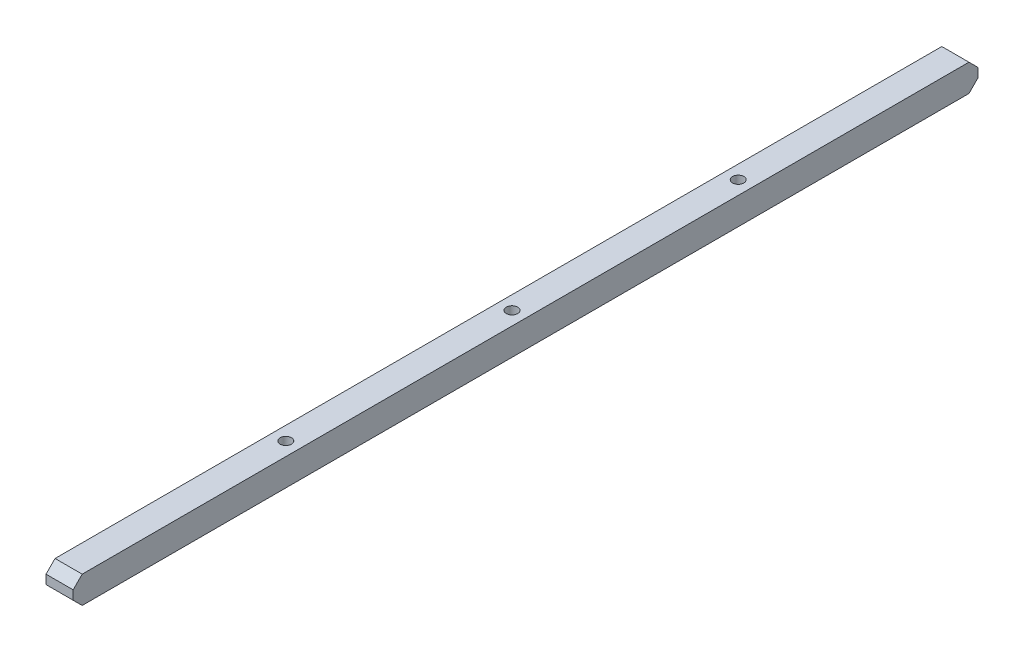
SolidWorks part; units mm, degrees
material "AISI 1045 钢，冷拔"
ref_plane "前视基准面" through (0, 0, 0) normal (0, 0, 1) x (1, 0, 0)
ref_plane "上视基准面" through (0, 0, 0) normal (0, 1, 0) x (1, 0, 0)
ref_plane "右视基准面" through (0, 0, 0) normal (1, 0, 0) x (0, 0, -1)
sketch "草图1" plane through (0, 0, 0) normal (0, 0, 1) x (1, 0, 0)
  line L1 (-3, 3) -> (3, 3)
  line L2 (-3, 3) -> (-3, -3)
  line L3 (-3, -3) -> (3, -3)
  line L4 (3, 3) -> (3, -3)
  line L5 (-3, 3) -> (3, -3) construction
  line L6 (-3, -3) -> (3, 3) construction
  point P0 (0, 0)
  dimension "D1" = 6
extrude "凸台-拉伸1" add sketch "草图1" along normal blind 200
sketch "草图2" plane through (0, 3, 0) normal (0, 1, 0) x (1, 0, 0)
  line L0 (0, 0) -> (0, -50) construction
  line L1 (0, -50) -> (0, -100) construction
  line L2 (0, -100) -> (0, -150) construction
  line L3 (0, -150) -> (0, -200) construction
  line L4 (3, -200) -> (-3, -200) construction
  dimension "D1" = 50
hole_wizard "M3 螺纹孔1" positions "3D草图1" profile "草图3" tap size "M3" standard "GB" end condition through all
sketch3d "3D草图1"
  point P0 (0, 3, 50)
  point P3 (0, 3, 100)
  point P6 (0, 3, 150)
sketch "草图3" plane through (0, 3, 50) normal (1, 0, 0) x (0, 0, 1)
  line L0 (0, 0) -> (0, 6)
  line L1 (0, 6) -> (1.25, 6)
  line L2 (1.25, 6) -> (1.25, 0)
  line L5 (1.25, 0) -> (0, 0)
  line L11 (0, -6.35) -> (0, 107.95) construction
  dimension "通孔螺纹孔钻头直径" = 2.5
  dimension "通孔螺纹孔钻头深度" = 6
cosmetic thread "孔螺蚊线1" parameters "D2"=3
cosmetic thread "孔螺蚊线2" parameters "D2"=3
cosmetic thread "孔螺蚊线3" parameters "D2"=3
chamfer "倒角1" distance 2 angle 45 4 edges at (0, -3, 0) (0, 3, 0) (0, -3, 200) (0, 3, 200)
